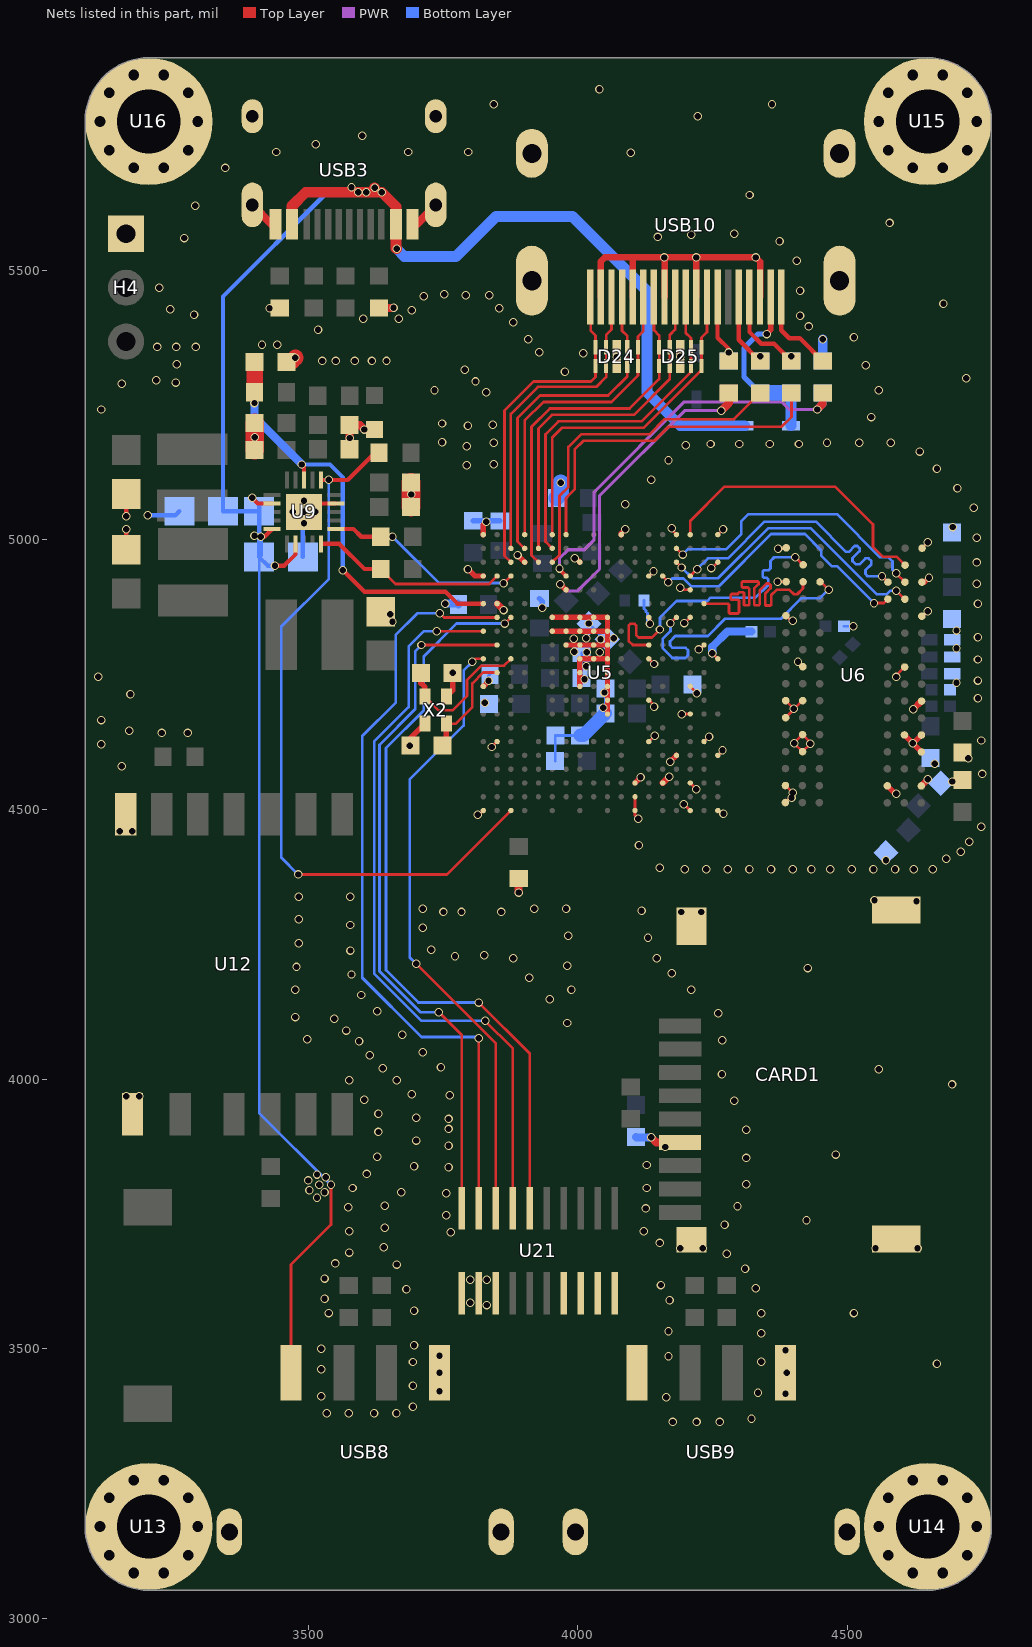
[diagram p0: the nets of this part, all layers, seen from the top]
# Altium PCB MISC105417.pcbdoc (part 3 of 5)
Units mil, origin at the board's own origin, x right, y up, seen from the top; angles counter-clockwise.
Board outline 1681.1 x 2842.52 mil, 4 copper layers (Top Layer, GND, PWR, Bottom Layer), stack 62.447 mil thick; 102 components, 152 nets, 737 pads, 611 vias.

## Via types
v1: diameter 15.7, hole 11.8, Top Layer to Bottom Layer, 611 vias

## Nets (pads, with @x,y where several pads share a name; then routed paths per layer and width w, separated by ;. In a path a pad name is that pad's centre, name@x,y a point inside that pad or via, vN(x,y) a via of type N, cw(c..) or ccw(c..) an arc to the next point about the centre after c; other vN are vias at no path point) (continued)
GND: C5.1 C12.1 C14.1 C15.1 C17.1 C18.1 C19.1 C22.1 C23.1 C24.1 C25.1 C26.1 C27.1 C94.2 C99.2 C100.1 C105.1 C106.1 C108.2 C116.1 C118.1 C120.1 C121.1 C122.1 C123.1 C124.1 C125.1 C126.1 C127.1 C128.1 C129.1 C132.2 C133.1 C136.2 C137.1 C138.2 C139.1 C140.1 C141.1 C143.1 C144.1 CARD1.6 CARD1.10 CARD1.11 CARD1.12 CARD1.13 D24.3 D24.8 D25.3 D25.8 H4.1 LED2.1 R6.2 R10.1 R11.1 R26.2 R43.2 R52.2 R56.2 R70.1 R84.1 R124.2 U5.A1 U5.A10 U5.A18 U5.A21 U5.B6 U5.B16 U5.D19 U5.F14 U5.F15 U5.G13 U5.G14 U5.G15 U5.H10 U5.H11 U5.H12 U5.H13 U5.H14 U5.H15 U5.H19 U5.J12 U5.J13 U5.J14 U5.J15 U5.K8 U5.K9 U5.K10 U5.K11 U5.K12 U5.K13 U5.K14 U5.K15 U5.L21 U5.M1 U5.M2 U5.M3 U5.N6 U5.N9 U5.N12 U5.N15 U5.N18 U5.P3 U5.R5 U5.R21 U5.T1 U5.T3 U5.T8 U5.T10 U5.T15 U5.T17 U5.U6 U5.U13 U5.V1 U5.V5 U5.V12 U5.V19 U5.V21 U6.A9 U6.B1 U6.B3 U6.B9 U6.D1 U6.D8 U6.E1 U6.E2 U6.E8 U6.F9 U6.G1 U6.G8 U6.G9 U6.J2 U6.J8 U6.M1 U6.M9 U6.P1 U6.P9 U6.T1 U6.T9 U9.9 U9.21 U12.7 U12.8 U13.1 U14.1 U15.1 U16.1 U21.1 U21.2 U21.3 USB3.12 USB3.13 USB3.14 USB3.15 USB3.A1B12 USB3.B1A12 USB8.4 USB8.5 USB8.6 USB9.4 USB9.5 USB9.6 USB10.2 USB10.5 USB10.8 USB10.11 USB10.17 USB10.20 X2.2 X2.4 | length 3790.7
  Top Layer w5: v1(3814,4490) 3816.39,4490 U5.A1@3824.48,4498.09 ; v1(3840,4616) U5.B6@3850.07,4626.05 ; U5.M2@4105.98,4523.69 U5.M1@4105.98,4498.09 4105.98,4489.17 v1(4112.2,4482.94) ; U5.N6@4131.57,4626.05 4142.2,4636.68 v1(4142.2,4636.94) ; U5.N9@4131.57,4702.82 4141.2,4693.19 v1(4141.2,4690.94) ; U5.N12@4131.57,4779.59 v1@4141.2,4769.96 ; U5.N15@4131.57,4856.36 4133.62,4854.31 v1(4133.62,4844.33) ; U5.N18@4131.57,4933.13 4140.2,4941.76 v1(4140.2,4941.94) ; v1(4174.2,5021.94) 4174.2,5018.46 U5.R21@4182.75,5009.91 ; v1(4189.91,4911.38) 4193.75,4907.54 U5.T17@4208.34,4907.54 ; v1(4192.35,4676.65) 4192.93,4677.23 U5.T8@4208.34,4677.23 ; v1(4196.2,4509.94) 4196.49,4509.94 U5.T1@4208.34,4498.09 ; v1(4197.2,4845.94) 4197.92,4845.94 U5.T15@4208.34,4856.36 ; U5.T3@4208.34,4549.28 4219.2,4538.42 v1(4219.2,4537.94) ; U5.T10@4208.34,4728.41 4220.2,4716.55 v1(4220.2,4715.94) ; v1(4224.2,4796.94) 4225.69,4796.94 U5.U13@4233.93,4805.18 ; U5.U6@4233.93,4626.05 4242.82,4634.94 v1(4243.2,4634.94) ; v1(4247.2,4947.94) 4248.74,4947.94 U5.V19@4259.52,4958.72 ; v1(4249.2,4789.94) U5.V12@4259.52,4779.59 ; U5.V1@4259.52,4498.09 4265.61,4492 v1(4270,4492) ; U5.V5@4259.52,4600.46 4268.2,4609.14 v1(4268.2,4609.94) ; U5.V21@4259.52,5009.91 4269.2,5019.59 v1(4269.2,5019.94) ; v1(4370.32,4922.36) 4385.97,4922.36 U6.P9@4386.14,4922.49 ; v1(4371.2,4983.94) 4384.79,4983.94 U6.T9@4386.34,4985.49 ; U6.A9@4384.84,4512.99 4393.78,4521.94 v1(4396.2,4521.94) ; U6.B9@4384.94,4544.49 4398.2,4531.23 v1(4398.2,4530.94) ; U6.F9@4385.34,4670.49 4385.54,4670.49 U6.G8@4416.94,4701.89 ; U6.G9@4385.44,4701.99 4400.2,4687.23 v1(4400.2,4686.94) ; U6.M9@4385.94,4859.49 4395.49,4849.94 v1(4398.2,4849.94) ; v1(4408.2,4773.94) 4408.2,4773.83 U6.J8@4417.14,4764.89 ; v1(4590.2,4745.94) 4590.2,4748.36 U6.J2@4606.14,4764.29 ; U6.M1@4637.94,4858.69 4639.94,4858.69 v1(4649.2,4867.94) ; U6.T1@4638.34,4984.69 4649.2,4995.56 v1(4649.2,4995.94) ; v1@4401.2,4622.83 U6.D8@4416.64,4607.39 v1(4431.2,4621.94) 4431.2,4624.43 U6.E8@4416.74,4638.89 4401.2,4623.36 v1(4401.2,4622.94) v1@4401.2,4622.83
  Top Layer w8: C136.2@3162.16,4981.84 v1(3162.16,5020) ; v1(3162.16,5044) C138.2@3162.16,5085.45 ; v1(3492,5052) 3507.7,5067.7 U9.9@3551.1,5067.7 ; D24.3@4072,5322.7 v1(4072,5339.46) D24.8@4072,5357.3 ; D25.3@4190,5322.7 v1(4190,5340.2) D25.8@4190,5357.3
  Top Layer w10: C94.2@3689.72,4618.45 3689.72,4632.96 X2.4@3716.12,4659.35 ; X2.2@3756.12,4709.35 3767.78,4721.01 v1(3767.78,4753.45) ; v1(3796,4946) 3808.87,4933.13 U5.A18@3824.48,4933.13 ; U5.A10@3824.48,4728.41 3834.2,4738.13 v1(3834.2,4738.94) ; U5.A21@3824.48,5009.91 3824.48,5028.48 v1(3830,5034) ; v1(3888,4972) U5.D19@3901.25,4958.72 ; U5.F14@3952.43,4830.77 U5.G14@3978.02,4830.77 U5.H14@4003.61,4830.77 U5.J14@4029.2,4830.77 U5.K14@4054.8,4830.77 ; U5.F15@3952.43,4856.36 U5.G15@3978.02,4856.36 U5.H15@4003.61,4856.36 U5.J15@4029.2,4856.36 U5.K15@4054.8,4856.36 U5.K14@4054.8,4830.77 ; U5.G13@3978.02,4805.18 U5.H13@4003.61,4805.18 U5.J13@4029.2,4805.18 U5.K13@4054.8,4805.18 ; v1(3994,4966) 3996.33,4966 U5.H19@4003.61,4958.72 ; U5.H10@4003.61,4728.41 U5.H11@4003.61,4754 U5.H12@4003.61,4779.59 U5.J12@4029.2,4779.59 U5.K12@4054.8,4779.59 ; U5.K8@4054.8,4677.23 U5.K9@4054.8,4702.82 U5.K10@4054.8,4728.41 U5.K11@4054.8,4754 U5.K12@4054.8,4779.59 ; U5.L21@4080.39,5009.91 4080.39,5012.39 v1(4088,5020) ; U5.M3@4105.98,4549.28 4116.2,4559.5 v1(4116.2,4559.94) ; v1(4171.2,4588.94) U5.R5@4182.75,4600.46 ; U6.B3@4573.94,4543.89 4588.89,4528.94 v1(4590.2,4528.94) ; U6.E2@4605.74,4638.29 v1(4621.39,4622.64) ; U6.D1@4637.14,4606.69 4637.14,4606.89 v1(4621.39,4622.64) ; U6.E1@4637.24,4638.19 4621.69,4622.64 v1(4621.39,4622.64) ; U6.P1@4638.14,4921.69 4642.95,4921.69 v1(4651.2,4929.94) ; U5.K12@4054.8,4779.59 U5.K13@4054.8,4805.18 ; U5.K13@4054.8,4805.18 U5.K14@4054.8,4830.77
  Top Layer w12: C137.1@3634.16,4866.84 3639,4862 v1(3652,4862) ; U5.B16@3850.07,4881.95 v1(3862,4870) ; USB10.2@4042.53,5450.93 4042.53,5516.52 4050,5524 4101.47,5524 ; USB10.5@4101.57,5450.93 4101.57,5523.9 4101.47,5524 ; U5.P3@4157.16,4549.28 4168.82,4560.94 v1(4169.2,4560.94) ; USB10.8@4160.64,5450.93 4160.64,5523.79 v1(4160.42,5524) ; USB10.11@4219.69,5450.93 4219.69,5523.89 v1(4219.57,5524) ; USB10.17@4337.8,5450.93 4338,5451.14 4338,5516 v1(4330,5524) v1(4219.57,5524) ; v1@4622.2,4685.96 U6.G1@4637.44,4701.19 ; U6.B1@4636.94,4543.69 v1(4649.2,4555.94) ; 4101.47,5524 v1(4160.42,5524) ; v1(4160.42,5524) v1(4219.57,5524)
  Top Layer w15: USB3.13@3396.1,5621.45 3432.1,5585.45 USB3.B1A12@3439.2,5585.45 ; C27.1@3576.53,5213 3595.41,5213 v1(3603.62,5204.79) LED2.1@3622.56,5204.79 ; C118.1@3576.69,5168.29 v1(3576.69,5189.09) C27.1@3576.69,5212.84 ; R70.1@3631.03,5430.42 v1(3658,5430.42) ; USB3.A1B12@3693.2,5585.45 3700.3,5585.45 USB3.12@3736.3,5621.45 ; v1(3890,4346) R52.2@3890,4372.34 ; v1(4136,3892) 4145.3,3882.7 CARD1.6@4189.4,3882.7
  Top Layer w30: C100.1@3459.53,5330 3468,5330 v1(3476,5338)
  Top Layer w35: C14.1@3400.47,5167 v1(3400.47,5190.79) C15.1@3400.47,5217 ; C5.1@3690.53,5061 v1(3690.53,5084.42) C12.1@3690.53,5107
  Bottom Layer w5: v1(3834.2,4738.94) 3834.2,4748.15 C132.2@3836.96,4750.91 ; C26.1@3957.68,4589.94 3958.2,4590.47 C24.1@3958.2,4637.46 C25.1@4004.25,4637.46 ; C23.1@4007.01,4743.94 C22.1@4007.01,4790.68 ; v1(4020.4,4845.03) 4049.61,4815.82 C124.1@4054.33,4815.82 ; C122.1@4050.95,4678.21 C126.1@4050.95,4724.21 ; R6.2@4122.52,4887.91 4122.52,4872.62 4126.2,4868.94 4126.2,4866.94 4129.2,4863.94 4129.2,4848.75 v1(4133.62,4844.33) ; R10.1@4493.24,4839.94 4510.28,4839.94 v1@4510.55,4839.67
  Bottom Layer w8: v1(3202,5046) 3253.32,5046 C140.1@3260.61,5053.29 ; C141.1@3489.74,4968.29 C139.1@3489.74,5053.29
  Bottom Layer w10: R26.2@3806,5035.66 v1@3830.85,5035.66 ; v1(3830,5034) 3830.85,5034.85 v1@3830.85,5035.66 ; C105.1@3855.2,5035.5 3855.05,5035.66 v1@3830.85,5035.66 ; C108.2@3928.52,4891.47 3934,4885.99 v1(3934,4874)
  Bottom Layer w15: v1@3658,5430 v1(3658,5430.42) ; v1(3754,4882) 3776.59,4882 C106.1@3778.64,4879.94 ; C133.1@4108,3892.47 4108.47,3892 v1(4136,3892) ; v1(4249.2,4789.94) 4249.2,4801.94 4277.2,4829.94 R11.1@4322.16,4829.94
  Bottom Layer w18: R124.2@4454,5331.66 v1(4454,5372)
  Bottom Layer w25: C25.1@4004.25,4637.46 4010.19,4637.46 C122.1@4050.95,4678.21
  Bottom Layer w30: R84.1@3960.54,5077.94 3968,5085.4 v1(3968,5106)
  other v1: 4176,3364 4220,3364 4263.31,3364 4322,3370 3534,3380 3574.98,3380 3621.88,3380 3663.4,3380 3694,3392 4164,3410 3524,3412 4385.1,3416.1 4334,3418 3743.37,3420.71 3694,3431.03 3743.37,3455.43 4387.43,3455.43 3524,3461.78 4666,3472 3694,3475.24 4340,3476 4168,3486.07 3743.37,3486.76 4385.1,3497.04 3524,3500 3696,3506 4340,3528.87 4168,3532 3538,3566 4340,3565.77 4512,3566 3696,3570.2 3831,3580.92 3800,3585.24 4170,3590 3530,3592.88 3682,3610 4330,3612 4154,3618 3800,3628 3831,3628 3530,3630 4310,3648 3664,3656 3550,3658 4276,3676 3576,3678.22 4190,3686 4231.49,3686 4552,3686 4630,3686 3640,3688 4152,3696 3764,3716 3576,3718 4122,3718 3642,3724 4272,3730 4424,3738 3756,3747.61 4126,3760 3574,3762 4296,3764 3642,3765.1 3756,3788 3672,3790 3582,3798 4128,3798 4312,3804.68 3608,3824 3760,3836.42 3696,3838 4128,3840.63 4312,3853.7 3628,3856 4478,3860 4162,3874 3760,3876.4 3700,3886 3630,3901.96 4312,3906 3760,3907.54 3760,3926 3700,3928.49 3630,3936 4290,3960 3604,3962 3162,3968 3186.4,3968 3762,3970 3692,3972 4694,3990 3576,3998 3664,3998 4267.21,4008.7 4558,4018 3638,4020 3746,4022 3614,4044 3712,4050 3594,4070 4268,4072 3498,4074 3674,4082 3570,4090 3980,4104 3548,4112 3476,4115.03 4260,4122 3628,4126 3948,4148 3598,4156 3476,4166 3988,4166 4210,4166 3910,4188 3580,4194 4174,4196 4426,4206 3478,4208 3980,4210 3880,4224 4146,4224 3772,4228 3826,4230 3578.1,4238.45 3728,4240 3482,4252.28 4130,4262 3982,4266 3712,4280.52 3578,4285.82 3482,4296.36 3750.6,4310 3784.05,4310 3858,4310 4192,4310 4228.68,4310 4118,4312 3712,4316 3918.98,4316 3978,4316 4628,4330 4550,4332 3482,4338 3578,4338 4198.2,4388.94 4238.2,4388.94 4278.2,4388.94 4318.2,4388.94 4358.2,4388.94 4398.2,4388.94 4433.2,4388.94 4468.2,4388.94 4508.2,4388.94 4548.2,4388.94 4588.2,4388.94 4623.2,4388.94 4658.2,4388.94 4152,4392 4571.41,4405.94 4683.2,4408.94 4710,4422 4113.2,4433.94 4726,4440 3150,4460 3173.19,4460 4748,4468 4694.2,4551.94 4750,4566 3154,4580 4662.2,4584.94 4724.2,4594.94 3687.76,4618.45 3116,4621.04 4748,4628 3228,4642 3276,4642 3168,4646 3116,4666 4622.2,4685.94 4047.2,4688.94 3827.2,4697.94 4742,4706.38 3170,4714 4049.2,4716.94 4702.2,4735.21 4742,4739.25 4012.2,4741.94 3110,4746 4015.2,4765.94 4141.2,4769.94 4742,4778.3 4016.2,4791.94 4040.2,4791.94 3993.2,4792.94 4702.2,4799.29 4042,4815.82 3992.2,4816.94 4015.2,4817.94 4066.2,4817.94 4742,4819.47 4702.2,4831.94 4510.55,4839.63 3656,4848 4742,4882 4740,4918.72 4740,4958.29 4740,5004 4694.94,5023.98 3492,5031.31 3471.31,5052 3512.69,5052 4734,5060 4088,5066 3492,5072.69 4704,5096 4136,5112 4666,5132 3794,5138.37 3844,5140.36 4168,5148 4634,5164 3794,5174 4200,5176 4246,5178 4299.27,5178 4355.59,5178 4410,5178 3844,5180 4462,5180 4522,5180 4580,5180 3748,5181.43 3796,5212 3842,5214 3748,5216 4544,5228 3116,5242 3830,5274 3734,5278 4558,5278 3154,5290 3254,5292 3810,5294 3218,5296 4720,5300 3976,5312 3790,5316 4534,5324 3256,5326 3526,5332 3550.67,5332 3586,5332 3618,5332 3644.94,5332 4010,5346 3928,5348 3220,5358 3254.94,5358 3291.08,5358 3414,5362 3442.1,5362 3908,5372 4512,5376 3518,5390 4428,5396 3880,5404 3602,5410 3667.6,5410 4412,5415.9 3288,5418 3692,5426 3244,5428 3428,5430 3854,5430 4678,5438 3714,5452 3792,5454 3835.47,5454 3752,5456 4412,5462 3223.29,5468 4406,5518 4374,5554 3270,5560 4148,5562 4210,5566 4290,5568 4578,5588 3290,5620 4318.38,5639.85 3346,5690 4098,5718 3440.43,5719.6 3685.22,5719.6 3796.8,5719.6 3514,5734 3600,5750 4222,5786 3844,5808 4360,5808 4040,5836
H5V: D26.1 R117.1 R122.1 USB10.18 | length 339.6
  Top Layer w10: v1(4350,5382) 4357.48,5389.48 USB10.18@4357.48,5450.93
  Bottom Layer w10: R122.1@4338,5272.34 4308,5302.34 4308,5356 4334,5382 v1(4350,5382)
  Bottom Layer w20: D26.1@4395.2,5212 R117.1@4395.2,5271.54
  Bottom Layer w30: R122.1@4338,5272.34 R117.1@4396,5272.34 R117.1@4395.2,5271.54
HCEC: R121.1 U5.G17 | length 575.5
  Top Layer w10: v1(3967.32,4917.92) 3967.64,4917.92 U5.G17@3978.02,4907.54
  Top Layer w15: v1(4266,5240) 4280,5254 R121.1@4280,5272.34
  PWR w6: v1(3967.32,4917.92) 3980.15,4905.09 3999.09,4905.09 4040,4946 4040,5082 4198,5240 v1(4266,5240)
HDCEC: R120.2 R121.2 USB10.13 | length 127.9
  Top Layer w8: USB10.13@4259.06,5450.93 4259.06,5374.94 4280,5354 R121.2@4280,5331.66
  other v1: 4280,5347.81
HDHPD: R119.2 USB10.19 | length 162.6
  Top Layer w8: USB10.19@4377.16,5450.93 4377.16,5388.84 4392,5374 4411.66,5374 R119.2@4454,5331.66
HDMI_0N: D25.2 D25.9 U5.E20 USB10.9 | length 660.7
  Top Layer w5: U5.E20@3926.84,4984.31 3926.84,5206.84 3952,5232 4104,5232 4170.3,5298.3 D25.2@4170.3,5322.7 D25.9@4170.3,5357.3 4170.3,5380.3 4180.31,5390.31 USB10.9@4180.31,5450.93
HDMI_0P: D25.1 D25.10 U5.E19 USB10.7 | length 686.2
  Top Layer w5: U5.E19@3926.84,4958.72 3914,4971.56 3914,5210 3948,5244 4096,5244 4150.6,5298.6 D25.1@4150.6,5322.7 D25.10@4150.6,5357.3 4150.6,5379.4 4140.94,5389.06 USB10.7@4140.94,5450.93
HDMI_1N: D24.5 D24.6 U5.D21 USB10.6 | length 606
  Top Layer w5: U5.D21@3901.25,5009.91 3901.25,5221.25 3936,5256 4062,5256 4111.4,5305.4 D24.5@4111.4,5322.7 D24.6@4111.4,5357.3 4111.4,5377.4 4121.27,5387.27 USB10.6@4121.27,5450.93
HDMI_1P: D24.4 D24.7 U5.D20 USB10.4 | length 634.4
  Top Layer w5: U5.D20@3901.25,4984.31 3888,4997.56 3888,5226 3930,5268 4056,5268 4091.7,5303.7 D24.4@4091.7,5322.7 D24.7@4091.7,5357.3 4091.7,5378.3 4081.89,5388.1 USB10.4@4081.89,5450.93
HDMI_2N: D24.2 D24.9 U5.C20 USB10.3 | length 607.2
  Top Layer w5: U5.C20@3875.66,4984.31 3875.66,5233.66 3926,5284 4034,5284 4052.3,5302.3 D24.2@4052.3,5322.7 D24.9@4052.3,5357.3 4052.3,5380.3 4062.2,5390.2 USB10.3@4062.2,5450.93
HDMI_2P: D24.1 D24.10 U5.C19 USB10.1 | length 633
  Top Layer w5: U5.C19@3875.66,4958.72 3864,4970.38 3864,5240 3918,5294 4024,5294 4032.6,5302.6 D24.1@4032.6,5322.7 D24.10@4032.6,5357.3 4032.6,5379.4 4024,5388 4024,5449.77 USB10.1@4022.84,5450.93
HDMI_CN: D25.5 D25.6 U5.F21 USB10.12 | length 648.8
  Top Layer w5: U5.F21@3952.43,5009.91 3952.43,5190.43 3970,5208 4121.77,5208 4229.4,5315.63 D25.5@4229.4,5322.7 D25.6@4229.4,5357.3 4229.4,5375.4 4239.38,5385.38 USB10.12@4239.38,5450.93
HDMI_CP: D25.4 D25.7 U5.F20 USB10.10 | length 677.6
  Top Layer w5: U5.F20@3952.43,4984.31 3940,4996.74 3940,5196 3964,5220 4117.74,5220 4209.7,5311.96 D25.4@4209.7,5322.7 D25.7@4209.7,5357.3 4209.7,5374.3 4200,5384 USB10.10@4200.01,5450.93
HDSCL: R122.2 R123.2 USB10.15 | length 135.7
  Top Layer w8: USB10.15@4298.43,5450.93 4298.43,5371.23 R123.2@4338,5331.66
  other v1: 4338,5340.5
HDSDA: R117.2 R118.2 USB10.16 | length 165.4
  Top Layer w8: USB10.16@4318.11,5450.93 4318.11,5385.89 4340,5364 4363.66,5364 R118.2@4396,5331.66
  other v1: 4396,5340.5
HHPD: R119.1 R124.1 U5.G18 | length 763
  Top Layer w8: v1(3965.82,4947.01) 3965.82,4945.33 U5.G18@3978.02,4933.13
  Top Layer w15: v1(4444,5242) 4454,5252 R119.1@4454,5272.34
  PWR w6: v1(3965.82,4947.01) 3965.82,4965.82 3982,4982 4012,4982 4030,5000 4030,5089 4197,5256 4378,5256 4392,5242 v1(4444,5242)
  Bottom Layer w15: v1(4444,5242) 4454,5252 R124.1@4454,5272.34
HSCL: R123.1 U5.F19 | length 623.1
  Top Layer w5: U5.F19@3952.43,4958.72 3966,4972.29 3966,5082 3982.35,5098.35 3982.35,5172.35 4006,5196 4132.73,5196 4160.73,5224 4289.66,5224 R123.1@4338,5272.34
HSDA: R118.1 U5.G21 | length 635.9
  Top Layer w5: U5.G21@3978.02,5009.91 3978.02,5078.02 3994,5094 3994,5168 4010,5184 4142,5184 4168,5210 4378,5210 4396,5228 R118.1@4396,5272.34
HXIN: C94.1 U5.B11 X2.1 | length 202.9
  Top Layer w5: X2.1@3756.12,4659.35 3773.61,4659.35 3804.2,4689.94 3804.2,4733.94 3824.26,4754 U5.B11@3850.07,4754
  Top Layer w10: C94.1@3748.78,4618.45 3756.12,4625.79 X2.1@3756.12,4659.35
HXOUT: C99.1 U5.C12 X2.3 | length 273.8
  Top Layer w5: X2.3@3716.12,4709.35 3741.52,4683.94 3767.2,4683.94 3794.2,4710.94 3794.2,4739.94 3821.2,4766.94 3863.01,4766.94 U5.C12@3875.66,4779.59
  Top Layer w10: C99.1@3708.73,4753.45 3708.73,4734.42 3716.12,4727.03 X2.3@3716.12,4709.35
IRQ: R53.2 U5.C1 U9.11 | length 1355.7
  Top Layer w5: v1(3481.04,4379.54) 3757.11,4379.54 U5.C1@3875.66,4498.09 ; v1(3538,5112) v1@3538.9,5111.1
  Top Layer w8: U9.11@3523.5,5111.1 3538.9,5111.1 3573.1,5111.1 3624,5162 R53.2@3631.34,5162
  Bottom Layer w5: v1(3481.04,4379.54) 3450,4410.58 3450,4840 3538,4928 v1(3538,5112)
LCD_BL: U5.C15 U21.16 | length 1420.1
  Top Layer w5: v1(3816,4142) 3910.69,4047.31 U21.16@3910.69,3760.55 ; v1(3864.2,4844.94) U5.C15@3875.66,4856.36
  Bottom Layer w5: v1(3816,4142) 3704,4142 3644,4202 3644,4614 3714,4684 3714,4784 3774.94,4844.94 v1(3864.2,4844.94)
LCD_CS: U5.A12 U21.18 | length 1150.4
  Top Layer w5: v1(3700,4214) 3847.7,4066.3 U21.18@3847.7,3760.55 ; v1(3804,4774) 3809.59,4779.59 U5.A12@3824.48,4779.59
  Bottom Layer w5: v1(3700,4214) 3688,4226 3688,4556 3788,4656 3788,4758 v1(3804,4774)
LCD_DC: U5.A14 U21.17 | length 1394
  Top Layer w5: v1(3738,4830.77) U5.A14@3824.48,4830.77 ; v1(3828,4108) 3879.2,4056.8 U21.17@3879.2,3760.55
  Bottom Layer w5: v1(3738,4830.77) 3714.77,4830.77 3686,4802 3686,4690 3622,4626 3622,4196 3710,4108 v1(3828,4108)
LCD_RST: U5.B15 U21.19 | length 1447.4
  Top Layer w5: v1(3744,4864) 3751.64,4856.36 U5.B15@3850.07,4856.36 ; v1(3816,4076) 3816.2,4075.8 U21.19@3816.2,3760.55
  Bottom Layer w5: v1(3744,4864) 3702,4864 3662,4824 3662,4698 3600,4636 3600,4188 3710,4078 3814,4078 v1(3816,4076)
LED: U5.B13 U21.20 | length 1300.3
  Top Layer w5: v1(3709.81,4805.18) U5.B13@3850.07,4805.18 ; v1(3742,4124) 3784.71,4081.29 U21.20@3784.71,3760.55
  Bottom Layer w5: v1(3709.81,4805.18) 3698,4793.37 3698,4686 3632,4620 3632,4200 3708,4124 v1(3742,4124)
PMU_SCK: R3.2 U5.C18 U9.6 | length 371.6
  Top Layer w5: R3.2@3634.34,5006 v1(3656,5006) ; v1(3862,4920) 3862.53,4920 U5.C18@3875.66,4933.13
  Top Layer w8: U9.6@3551.1,5020.5 3583.5,5020.5 3598,5006 R3.2@3634.34,5006
  Bottom Layer w5: v1(3656,5006) 3742,4920 v1(3862,4920)
PMU_SDA: R2.2 U5.B18 U9.5 | length 363.4
  Top Layer w5: R2.2@3634.34,4946 3661.84,4918.5 3835.44,4918.5 U5.B18@3850.07,4933.13
  Top Layer w8: U9.5@3523.5,4992.9 3557.1,4992.9 3604,4946 R2.2@3634.34,4946
PS: C139.2 C140.2 C141.2 D26.2 U9.2 U9.17 U9.20 U21.7 U21.8 U21.9 U21.10 USB3.A4B9 USB3.B4A9 USB8.1 USB9.1 | length 4007.7
  Top Layer w5: USB8.1@3467.78,3455.43 3467.78,3655.78 3542,3730 v1(3542,3804)
  Top Layer w8: v1(3396,5078) 3406.2,5067.8 U9.17@3432.9,5067.8 ; v1(3412,5006) 3418.4,5006 U9.20@3432.9,5020.5 ; v1(3438,4952) 3455.05,4952 3476.2,4973.15 U9.2@3476.2,4992.9
  Top Layer w20: USB3.B4A9@3469.7,5585.45 3469.7,5619.7 3495,5645 v1(3592.47,5645) v1(3607.05,5645) 3622.83,5645 ; v1@3622.83,5652.83 3622.83,5645 ; v1(3664,5540) 3662.7,5541.3 USB3.A4B9@3662.7,5585.45 3663,5585.74 3663,5618 v1(3636,5645) 3622.83,5645
  Bottom Layer w5: C141.2@3408.64,4968.29 3408.64,3937.36 v1(3542,3804)
  Bottom Layer w8: v1(3396,5078) 3408.64,5065.36 C139.2@3408.64,5053.29 ; v1(3412,5006) 3412,4971.65 C141.2@3408.64,4968.29 ; v1(3438,4952) 3424.93,4952 C141.2@3408.64,4968.29 ; v1(3592.47,5645) 3535,5645 3341.71,5451.71 C140.2@3341.71,5053.29 C139.2@3408.64,5053.29 ; C141.2@3408.64,4968.29 C139.2@3408.64,5053.29
  Bottom Layer w20: v1(3664,5540) 3678,5526 3774,5526 3848,5600 3990,5600 4128,5462 4128,5274 4190,5212 D26.2@4308.8,5212
  other v1: 3516,3780.1 3530,3790 3502,3794 3520,3804 3500,3812 3532,3818 3516,3822.94 3400,5008 3623,5653 3580,5654
RESET: C100.2 R49.1 U5.A16 U9.13 | length 781.2
  Top Layer w8: v1(3488,5140) 3492,5136 U9.13@3492,5111.1 ; v1(3564,4944) 3604,4904 3754.42,4904 3776.47,4881.95 U5.A16@3824.48,4881.95
  Top Layer w30: R49.1@3400.34,5274 3400.47,5274.13 C100.2@3400.47,5330
  Bottom Layer w8: v1(3488,5140) 3540,5140 3564,5116 v1(3564,4944)
  Bottom Layer w15: v1(3400,5254) 3400,5228 v1(3488,5140)
SA0: U5.P18 U6.N3 | length 535
  Top Layer w5: U5.P18@4157.16,4933.13 4167.43,4922.86 v1(4167.43,4921.28) ; v1(4549.2,4882.94) 4567.59,4882.94 U6.N3@4575.04,4890.39
  Bottom Layer w5: v1(4167.43,4921.28) 4174.68,4928.54 4195.75,4928.54 4210.34,4913.94 4261.2,4913.94 4358.2,5010.94 4421.2,5010.94 4451.2,4980.94 4451.2,4970.77 4470.62,4951.35 4480.79,4951.35 v1(4549.2,4882.94)
SA1: U5.R15 U6.P7 | length 535
  Top Layer w5: v1@4171.64,4845.71 4182.29,4856.36 U5.R15@4182.75,4856.36 ; U6.P7@4449.14,4922.29 4450.85,4922.29 v1(4465.2,4907.94)
  Bottom Layer w5: v1(4171.68,4845.71) 4171.68,4830.86 4157.2,4816.37 4157.2,4799.2 4175.24,4781.16 4199.23,4781.16 4204.22,4786.15 4204.22,4795.7 4199.96,4799.96 4175.66,4799.96 4170.63,4804.99 4170.63,4812.06 4180.51,4821.94 4241.2,4821.94 4273.13,4853.87 4376.63,4853.87 4414.7,4891.94 4449.2,4891.94 v1(4465.2,4907.94)
SA2: U5.T18 U6.P3 | length 535
  Top Layer w5: U5.T18@4208.34,4933.13 v1(4221.2,4945.94) ; v1(4564.04,4932.69) 4564.34,4932.69 U6.P3@4575.14,4921.89
  Bottom Layer w5: v1(4221.2,4945.94) 4241.2,4965.94 4278.2,4965.94 4346.2,5033.94 4441.2,5033.94 4497.2,4977.94 4502.51,4977.94 4513.22,4988.66 4518.47,4988.66 4522.58,4984.55 4522.58,4979.59 4509.45,4966.47 4509.45,4960.69 4515.44,4954.71 4522.03,4954.71 4533.27,4965.94 4539.2,4965.94 4544.2,4960.94 4544.2,4954.94 4533.37,4944.11 4533.37,4936.78 4537.46,4932.69 v1(4564.04,4932.69)
SA3: U5.R19 U6.N2 | length 535
  Top Layer w5: U5.R19@4182.75,4958.72 4192.2,4949.27 v1(4192.2,4948.94) ; v1(4590.2,4905.94) 4605.86,4890.29 U6.N2@4606.54,4890.29
  Bottom Layer w5: v1(4192.2,4948.94) 4212.2,4928.94 4260.2,4928.94 4353.2,5021.94 4431.66,5021.94 4554.5,4899.1 4572.8,4899.1 4579.64,4905.94 v1(4590.2,4905.94)
SA4: U5.U16 U6.P8 | length 535
  Top Layer w5: U5.U16@4233.94,4881.94 4278.41,4881.94 4280.2,4880.14 4280.2,4864.83 4281.41,4863.63 4296.85,4863.63 4298.61,4865.39 4298.61,4887.7 4296.97,4889.33 4284.74,4889.33 4283.2,4890.87 4283.2,4898.25 4284.84,4899.89 4296.24,4899.89 4299.55,4903.21 4305.96,4903.21 4308.24,4900.93 4308.24,4879.92 4309.49,4878.67 4315.96,4878.67 4317.58,4880.29 4317.58,4909.63 4315.28,4911.94 4305.36,4911.94 4303.81,4913.49 4303.81,4921.3 4305.45,4922.94 4333.34,4922.96 4335.35,4920.95 4335.35,4918.31 4327,4909.97 4327,4880.5 4328.56,4878.94 4335.47,4878.94 4337.09,4880.56 4337.09,4906.12 4350.17,4919.2 4354.29,4919.2 4357.08,4916.42 4357.08,4910.5 4347.43,4900.85 4347.43,4879.69 4348.64,4878.49 4357.21,4878.49 4358.6,4879.87 4358.6,4897.63 4368.56,4907.59 4392.17,4907.59 4400.46,4899.31 4406.86,4899.31 4417.64,4910.08 U6.P8@4417.64,4922.39
SA5: U5.R20 U6.P2 | length 535
  Top Layer w5: U5.R20@4182.75,4984.31 v1@4194.12,4972.94 ; v1(4590.2,4937.94) 4606.36,4921.79 U6.P2@4606.64,4921.79
  Bottom Layer w5: v1(4194.2,4972.94) 4204.2,4982.94 4275.2,4982.94 4303.09,5010.82 4303.09,5034.82 4316.2,5047.94 4480.2,5047.94 4560.26,4967.89 4575.81,4967.89 4583.37,4960.33 4583.37,4944.78 v1(4590.2,4937.94)
SA6: U5.N13 U6.R8 | length 535
  Top Layer w5: U5.N13@4131.57,4805.18 4101.97,4805.18 4094.2,4812.94 4094.2,4841.18 4097.41,4844.38 4105.23,4844.38 4108.03,4841.59 4108.03,4823.54 4112.62,4818.94 4137.2,4818.94 v1(4152.2,4833.94) ; v1(4403.2,4967.94) 4403.69,4967.94 U6.R8@4417.74,4953.89
  Bottom Layer w5: v1(4152.2,4833.94) 4152.2,4855.94 4183.2,4886.94 4240.33,4886.94 4246.33,4892.94 4329.2,4892.94 4353.2,4916.94 4353.2,4926.69 4349.95,4929.94 4345.12,4929.94 4343.12,4931.94 4343.12,4941.94 4345.12,4943.94 4353.93,4943.94 4357.19,4947.2 4357.19,4960.92 4364.2,4967.94 v1(4403.2,4967.94)
SA7: U5.T21 U6.R2 | length 535
  Top Layer w5: U5.T21@4208.34,5009.91 4208.34,5035.08 4272.2,5098.94 4477.2,5098.94 4547.2,5028.94 4547.2,4986.94 4565.2,4968.94 4591.09,4968.94 U6.R2@4606.74,4953.29